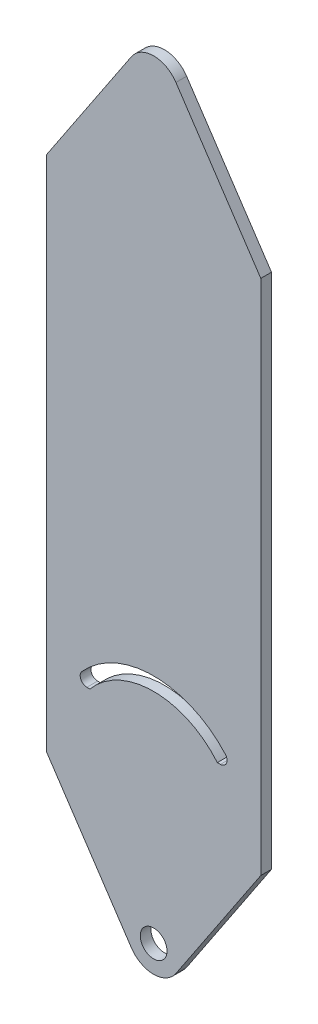
from build123d import *

# Parameters (mm, degrees)
SKETCH2_R           = 10
BOSS_EXTRUDE1_DEPTH = 8
CUT_EXTRUDE1_DEPTH  = 10


with BuildPart() as part:
    # Sketch2 → Boss-Extrude1 (new body)
    with BuildSketch(Plane.XY):
        with BuildLine():
            Line((-16.639082443, 618.903111451), (-80, 713.908799417))
            Line((-80, 713.908799417), (-80, 1100.091200583))
            Line((-80, 1100.091200583), (-16.639082443, 1195.096888549))
            ThreePointArc((-16.639082443, 1195.096888549), (0, 1204), (16.639082443, 1195.096888549))
            Line((16.639082443, 1195.096888549), (80, 1100.091200583))
            Line((80, 1100.091200583), (80, 713.908799417))
            Line((80, 713.908799417), (16.639082443, 618.903111451))
            ThreePointArc((16.639082443, 618.903111451), (0, 610), (-16.639082443, 618.903111451))
        make_face()
        with Locations((0, 630)):
            Circle(SKETCH2_R, mode=Mode.SUBTRACT)
    extrude(amount=BOSS_EXTRUDE1_DEPTH)

    # Sketch4 → Cut-Extrude1 (cut)
    with BuildSketch(Plane.XY.offset(8)):
        with BuildLine():
            Line((-49.84926833, 770.742207295), (-47.561478164, 770.742207295))
            ThreePointArc((-47.561478164, 770.742207295), (0, 793.027742088), (47.561478164, 770.742207295))
            Line((47.561478164, 770.742207295), (49.84926833, 770.742207295))
            ThreePointArc((49.84926833, 770.742207295), (54.413886924, 773.70155615), (53.575185994, 779.076504457))
            ThreePointArc((53.575185994, 779.076504457), (0, 803.027742088), (-53.575185994, 779.076504457))
            ThreePointArc((-53.575185994, 779.076504457), (-54.413886924, 773.70155615), (-49.84926833, 770.742207295))
        make_face()
    extrude(amount=-CUT_EXTRUDE1_DEPTH, mode=Mode.SUBTRACT)


solid = part.part
